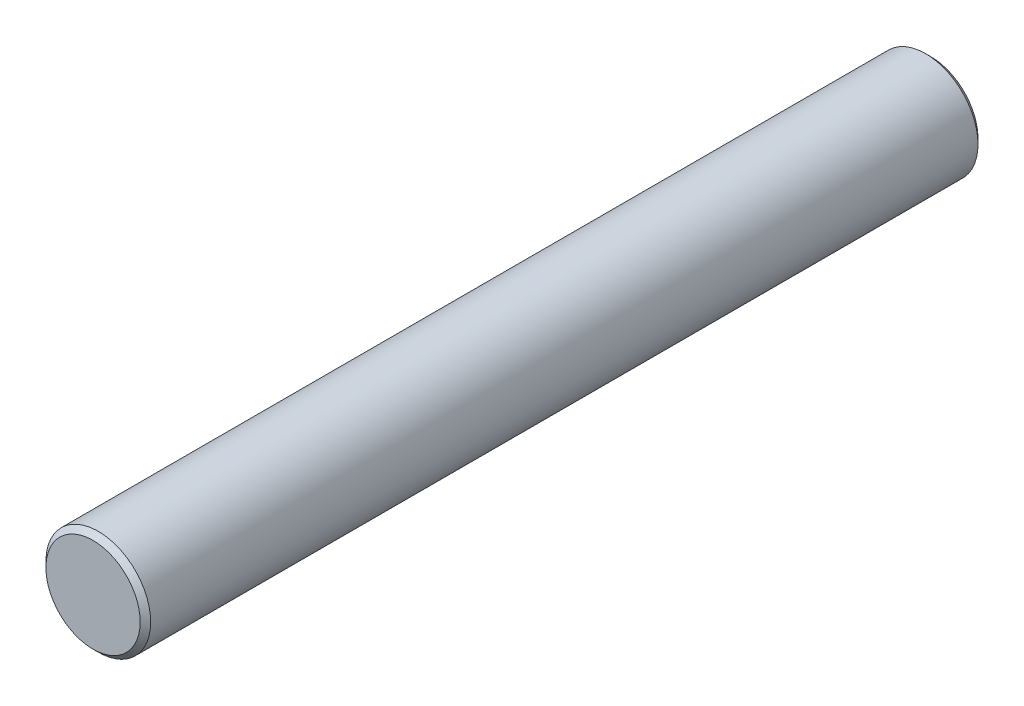
SolidWorks part; units mm, degrees
ref_plane "Front" through (0, 0, 0) normal (0, 0, 1) x (1, 0, 0)
ref_plane "Top" through (0, 0, 0) normal (0, 1, 0) x (1, 0, 0)
ref_plane "Right" through (0, 0, 0) normal (1, 0, 0) x (0, 0, -1)
sketch "草图1" plane through (0, 0, 0) normal (0, 0, 1) x (1, 0, 0)
  circle A0 centre (0, 0) radius 5
  dimension "D1" = 10
extrude "凸台-拉伸1" add sketch "草图1" along normal blind 80
chamfer "倒角1" distance 0.5 angle 45 2 edges at (5, 0, 0) (5, 0, 80)
